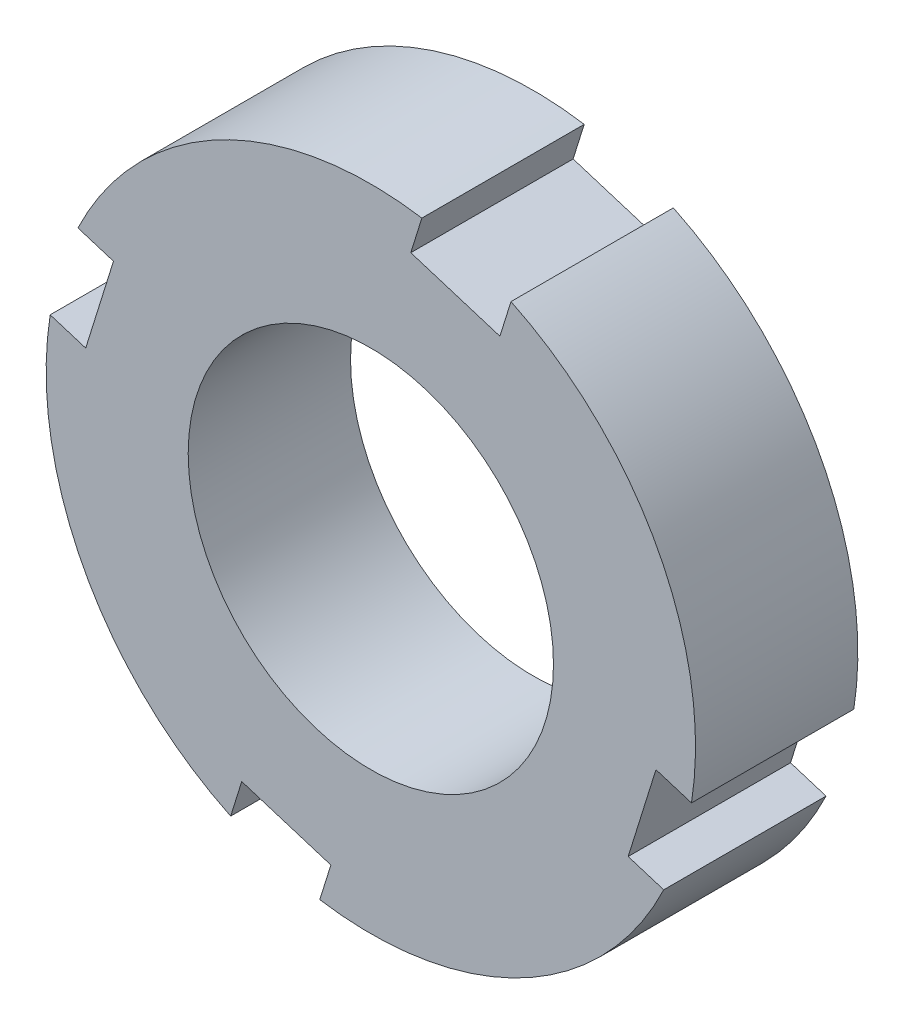
from build123d import *

# Parameters (mm, degrees)
SKETCH1_R           = 22.5
BOSS_EXTRUDE1_DEPTH = 20


with BuildPart() as part:
    # Sketch1 → Boss-Extrude1 (new body)
    with BuildSketch(Plane.XY.offset(-1549.998443067)):
        with BuildLine():
            Line((526.153967379, 269.86978568), (527.517933611, 274.246748006))
            ThreePointArc((527.517933611, 274.246748006), (502.642081617, 270.162396725), (485.149256781, 252.010509299))
            Line((485.149256781, 252.010509299), (489.526219107, 250.646543068))
            Line((489.526219107, 250.646543068), (486.104820559, 239.667288449))
            Line((486.104820559, 239.667288449), (481.727858233, 241.031254681))
            ThreePointArc((481.727858233, 241.031254681), (485.812209514, 216.155402687), (503.964096939, 198.662577851))
            Line((503.964096939, 198.662577851), (505.328063171, 203.039540177))
            Line((505.328063171, 203.039540177), (516.307317789, 199.618141629))
            Line((516.307317789, 199.618141629), (514.943351558, 195.241179303))
            ThreePointArc((514.943351558, 195.241179303), (539.819203552, 199.325530584), (557.312028388, 217.47741801))
            Line((557.312028388, 217.47741801), (552.935066061, 218.841384241))
            Line((552.935066061, 218.841384241), (556.35646461, 229.82063886))
            Line((556.35646461, 229.82063886), (560.733426936, 228.456672628))
            ThreePointArc((560.733426936, 228.456672628), (556.649075655, 253.332524622), (538.497188229, 270.825349458))
            Line((538.497188229, 270.825349458), (537.133221997, 266.448387132))
            Line((537.133221997, 266.448387132), (526.153967379, 269.86978568))
        make_face()
        with Locations(Location((521.230642584, 234.743963655, 0), (0, 0, 180))):
            Circle(SKETCH1_R, mode=Mode.SUBTRACT)
    extrude(amount=-BOSS_EXTRUDE1_DEPTH)


solid = part.part
